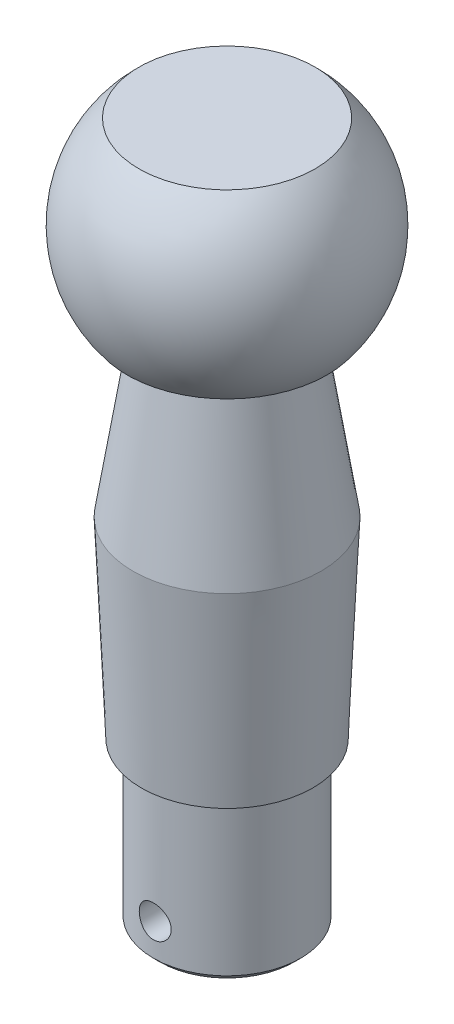
from build123d import *

# Parameters (mm, degrees)
CHAMFER_1_SIZE           = 1
FILLET_1_R               = 2
CUT_EXTRUDE_1_DEPTH      = 99.642029582
CUT_EXTRUDE_1_DEPTH_BACK = 99.642029582
SKETCH_3_R               = 2.5


with BuildPart() as part:
    # 草图1 → 旋转1 (revolve)
    with BuildSketch(Plane.XY, mode=Mode.PRIVATE) as revolve_1_sk:
        with BuildLine():
            Line((0, 14.5), (13.774977314, 14.5))
            ThreePointArc((13.774977314, 14.5), (19.953843795, 1.357982993), (15.612494996, -12.5))
            Line((15.612494996, -12.5), (10.5, -12.5))
            Line((10.5, -12.5), (14.7, -39.5))
            Line((14.7, -39.5), (13.4, -69.5))
            Line((13.4, -69.5), (11.5, -69.5))
            Line((11.5, -69.5), (11.5, -94.5))
            Line((11.5, -94.5), (0, -94.5))
            Line((0, -94.5), (0, -12.5))
            Line((0, -12.5), (0, 14.5))
        make_face()
    revolve(revolve_1_sk.sketch.rotate(Axis((0, 41.043678396, 0), (0, -1, 0)), 90), axis=Axis((0, 41.043678396, 0), (0, -1, 0)))

    # 倒角1
    chamfer_1_edges = [part.edges().sort_by_distance(p)[0] for p in [
        (0, -94.5, -11.5),
    ]]
    chamfer(chamfer_1_edges, length=CHAMFER_1_SIZE)

    # 圆角1
    fillet_1_edges = [part.edges().sort_by_distance(p)[0] for p in [
        (0, -12.5, -10.5),
    ]]
    fillet(fillet_1_edges, radius=FILLET_1_R)

    # 草图3 → 切除-拉伸1 (cut, two sides: drawn at the far end of the back side and taken through both)
    with BuildSketch(Plane.XY.offset(-CUT_EXTRUDE_1_DEPTH_BACK)):
        with Locations((0, -88.5)):
            Circle(SKETCH_3_R)
    extrude(amount=CUT_EXTRUDE_1_DEPTH + CUT_EXTRUDE_1_DEPTH_BACK, mode=Mode.SUBTRACT)


solid = part.part
